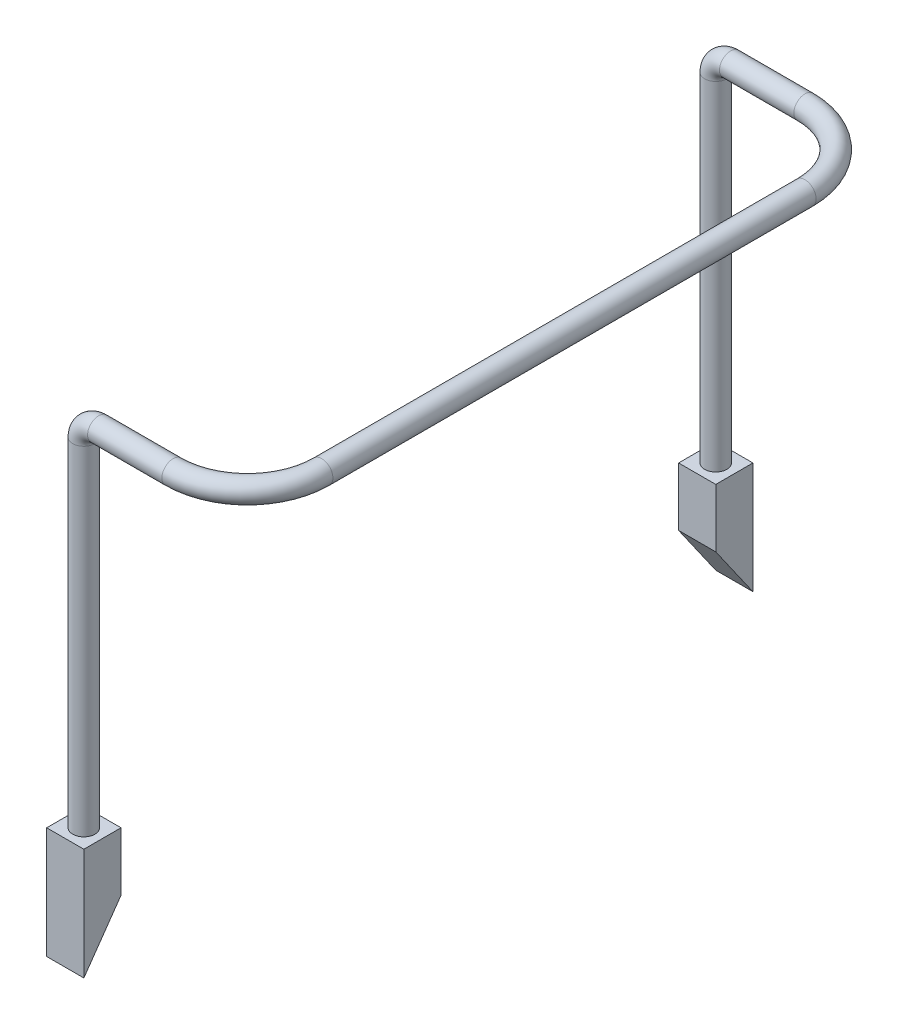
from build123d import *

# Parameters (mm, degrees)
SKETCH2_R               = 0.3
SKETCH4_W               = 1
SKETCH4_H               = 1
BOSS_EXTRUDE1_DEPTH     = 3
CUT_EXTRUDE1_DEPTH      = 23.185130234
CUT_EXTRUDE1_DEPTH_BACK = 23.185130234


with BuildPart() as part:
    # Sweep1: sweep along a curve in space
    with BuildLine() as sweep1_path:
        Line((0, 0, 0), (0, 12.1, 0))
        ThreePointArc((0, 12.1, 0), (0.117157288, 12.382842712, 0), (0.4, 12.5, 0))
        Line((0.4, 12.5, 0), (2.4, 12.5, 0))
        ThreePointArc((2.4, 12.5, 0), (3.814213562, 12.5, -0.585786438), (4.4, 12.5, -2))
        Line((4.4, 12.5, -2), (4.4, 12.5, -15))
        ThreePointArc((4.4, 12.5, -15), (3.814213562, 12.5, -16.414213562), (2.4, 12.5, -17))
        Line((2.4, 12.5, -17), (0.4, 12.5, -17))
        ThreePointArc((0.4, 12.5, -17), (0.117157288, 12.382842712, -17), (0, 12.1, -17))
        Line((0, 12.1, -17), (0, 0, -17))
    # Sketch2 → Sweep1 (sweep)
    with BuildSketch(Plane(origin=(0, 0, 0), x_dir=(1, 0, 0), z_dir=(0, 1, 0))):
        Circle(SKETCH2_R)
    sweep(path=sweep1_path.line)

    # Sketch4 → Boss-Extrude1 (add)
    with BuildSketch(Plane(origin=(0, 0, 0), x_dir=(-1, 0, 0), z_dir=(0, -1, 0))):
        with Locations((0, 17)):
            Rectangle(SKETCH4_W, SKETCH4_H)
        Rectangle(SKETCH4_W, SKETCH4_H)
    extrude(amount=-BOSS_EXTRUDE1_DEPTH)

    # Sketch5 → Cut-Extrude1 (cut, two sides: drawn at the far end of the back side and taken through both)
    with BuildSketch(Plane(origin=(0, 0, 0), x_dir=(0, 0, -1), z_dir=(1, 0, 0)).offset(-CUT_EXTRUDE1_DEPTH_BACK)):
        Polygon((-0.5, 0), (1.563257824, 2.946637548), (15.436742176, 2.946637548), (17.5, 0), align=None)
    extrude(amount=CUT_EXTRUDE1_DEPTH + CUT_EXTRUDE1_DEPTH_BACK, mode=Mode.SUBTRACT)


solid = part.part
